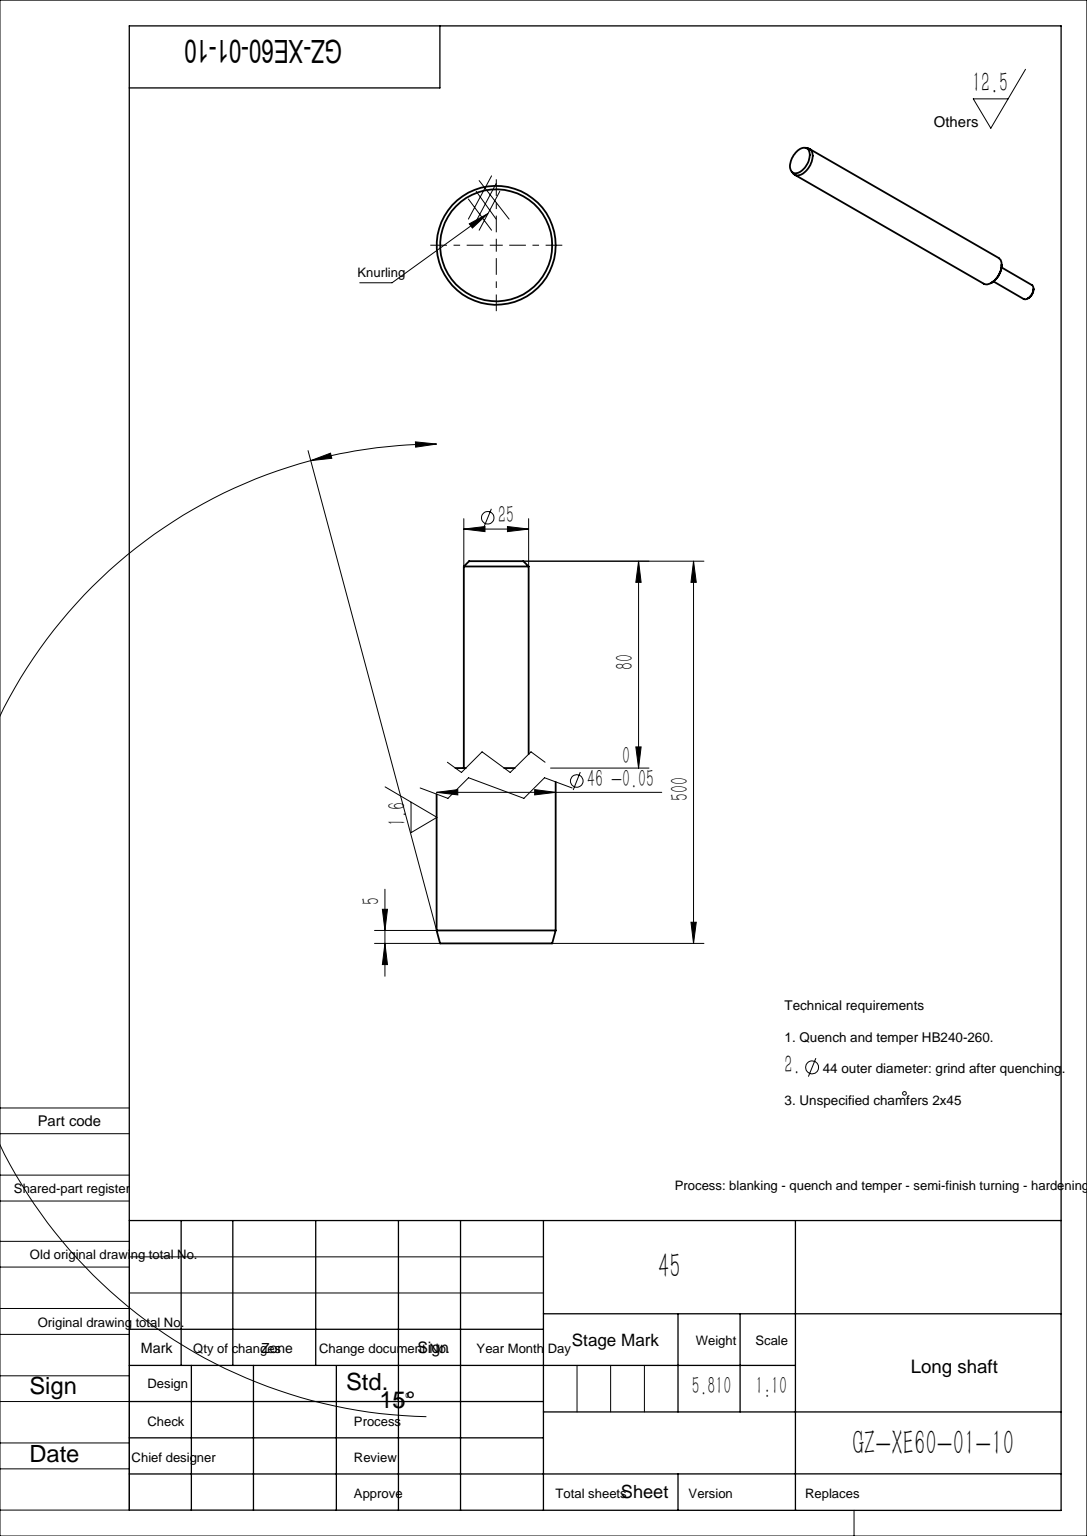
SolidWorks part; units mm, degrees
material "45"
ref_plane "Front Plane" through (0, 0, 0) normal (0, 0, 1) x (1, 0, 0)
ref_plane "Top Plane" through (0, 0, 0) normal (0, 1, 0) x (1, 0, 0)
ref_plane "Right Plane" through (0, 0, 0) normal (1, 0, 0) x (0, 0, -1)
sketch "Sketch1" plane through (0, 0, 0) normal (0, 0, 1) x (1, 0, 0)
  circle A0 centre (0, 0) radius 23
  dimension "D1" = 46
extrude "Boss-Extrude1" add sketch "Sketch1" along normal blind 420
chamfer "Chamfer1" distance 5 angle 15 1 edges at (23, 0, 420)
sketch "Sketch2" plane through (0, 0, 0) normal (0, 0, -1) x (-1, 0, 0)
  circle A0 centre (0, 0) radius 12.5
  dimension "D1" = 25
extrude "Boss-Extrude2" add sketch "Sketch2" along normal blind 80
chamfer "Chamfer2" distance 2 angle 45 2 edges at (23, 0, 0) (-12.5, 0, -80)
